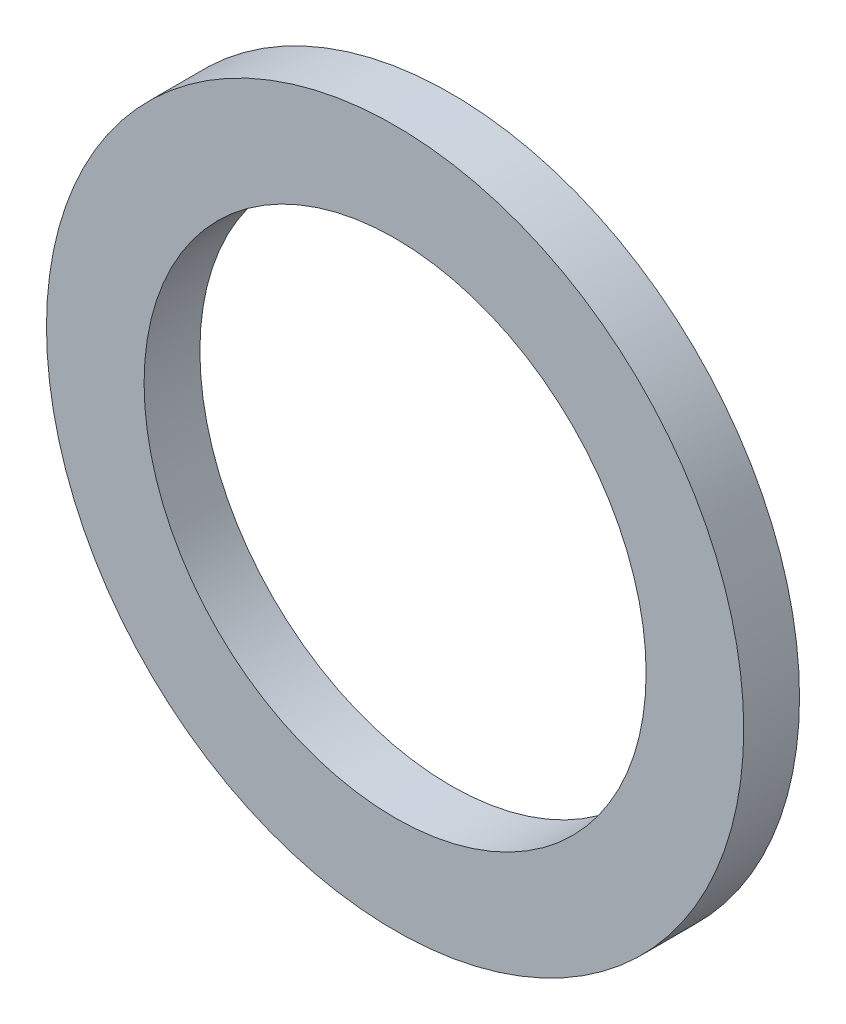
SolidWorks part; units mm, degrees
ref_plane "前视基准面" through (0, 0, 0) normal (0, 0, 1) x (1, 0, 0)
ref_plane "上视基准面" through (0, 0, 0) normal (0, 1, 0) x (1, 0, 0)
ref_plane "右视基准面" through (0, 0, 0) normal (1, 0, 0) x (0, 0, -1)
sketch "草图1" plane through (0, 0, 0) normal (0, 0, 1) x (1, 0, 0)
  circle A0 centre (0, 0) radius 18
  circle A1 centre (0, 0) radius 25
  dimension "D1" = 36
  dimension "D2" = 50
extrude "凸台-拉伸1" add sketch "草图1" along normal blind 4
